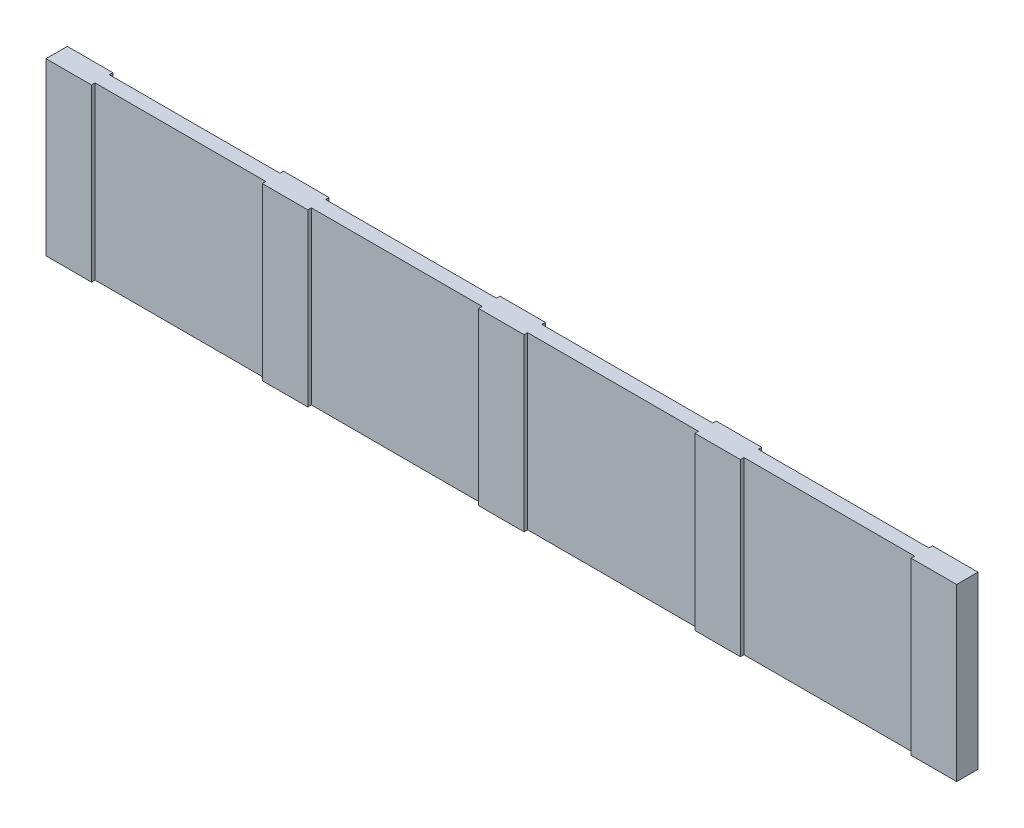
SolidWorks part; units mm, degrees
ref_plane "Front Plane" through (0, 0, 0) normal (0, 0, 1) x (1, 0, 0)
ref_plane "Top Plane" through (0, 0, 0) normal (0, 1, 0) x (1, 0, 0)
ref_plane "Right Plane" through (0, 0, 0) normal (1, 0, 0) x (0, 0, -1)
sketch "Sketch1" plane through (0, 0, 0) normal (0, 0, 1) x (1, 0, 0)
  line L1 (0, 0) -> (1270, 0)
  line L2 (0, 0) -> (0, 240)
  line L3 (0, 240) -> (1270, 240)
  line L4 (1270, 0) -> (1270, 240)
extrude "Boss-Extrude1" add sketch "Sketch1" along normal blind 20
sketch "Sketch3" plane through (0, 0, 0) normal (0, -1, 0) x (1, 0, 0)
  line L1 (0, -5) -> (64, -5)
  line L2 (0, -5) -> (0, 25)
  line L3 (0, 25) -> (64, 25)
  line L4 (64, -5) -> (64, 25)
  line L6 (0, 20) -> (1270, 20) construction
  line L8 (304, 25) -> (368, 25)
  line L9 (304, 25) -> (304, -5)
  line L10 (304, -5) -> (368, -5)
  line L11 (368, 25) -> (368, -5)
  line L13 (608, 25) -> (672, 25)
  line L14 (608, 25) -> (608, -5)
  line L15 (608, -5) -> (672, -5)
  line L16 (672, 25) -> (672, -5)
  line L18 (912, 25) -> (976, 25)
  line L19 (912, 25) -> (912, -5)
  line L20 (912, -5) -> (976, -5)
  line L21 (976, 25) -> (976, -5)
  line L23 (1216, 25) -> (1280, 25)
  line L24 (1216, 25) -> (1216, -5)
  line L25 (1216, -5) -> (1280, -5)
  line L26 (1280, 25) -> (1280, -5)
  point P11 (608, 25)
  point P16 (912, 25)
  point P21 (1216, 25)
  dimension "D1" = 240
  dimension "D2" = 5
  dimension "D3" = 240
  dimension "D4" = 240
  dimension "D5" = 240
extrude "Boss-Extrude2" add sketch "Sketch3" against normal up to vertex (240 mm away)
